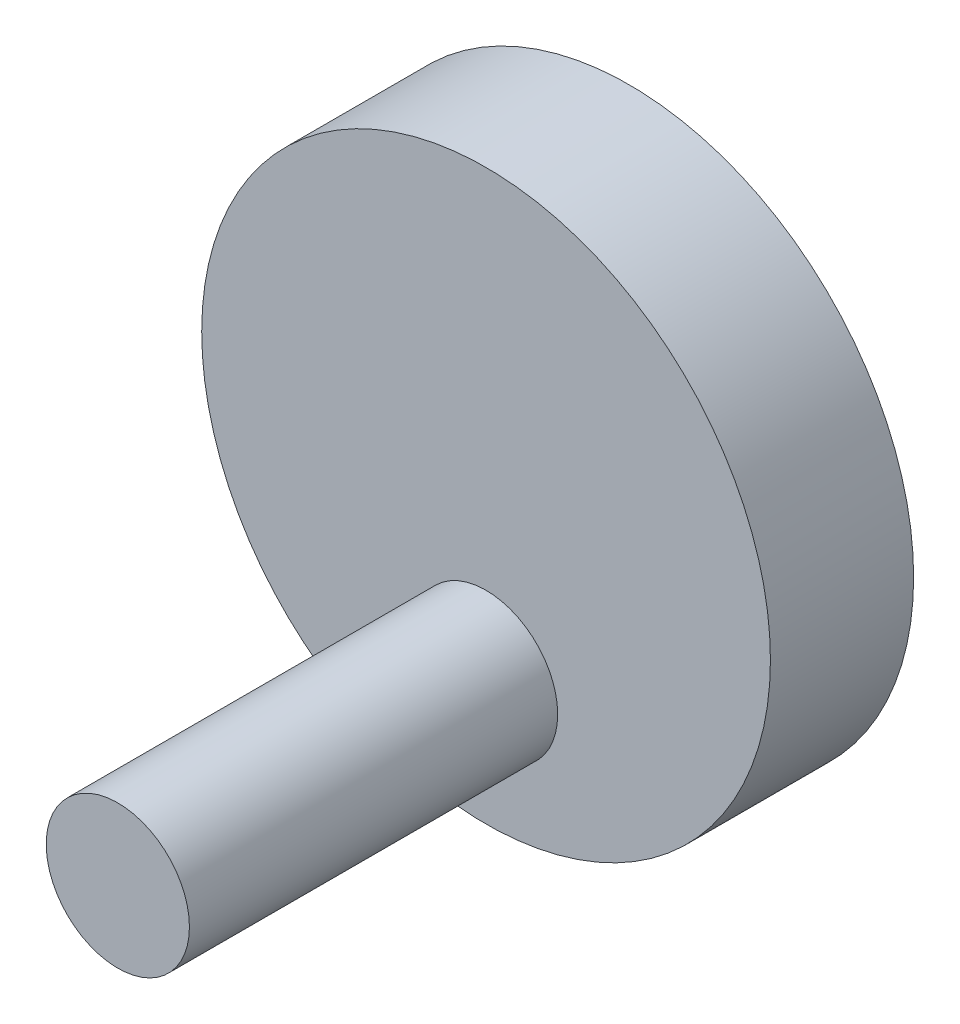
SolidWorks part; units mm, degrees
ref_plane "Front Plane" through (0, 0, 0) normal (0, 0, 1) x (1, 0, 0)
ref_plane "Top Plane" through (0, 0, 0) normal (0, 1, 0) x (1, 0, 0)
ref_plane "Right Plane" through (0, 0, 0) normal (1, 0, 0) x (0, 0, -1)
sketch "Sketch1" plane through (0, 0, 0) normal (0, 0, 1) x (1, 0, 0)
  circle A3 centre (0.6135, -35) radius 13.9
  circle A4 centre (0.6135, -35) radius 13.9
  dimension "D1" = 10
extrude "Boss-Extrude1" add sketch "Sketch1" against normal blind 5 and the other way blind 2
sketch "Sketch2" plane through (0, 0, -5) normal (0, 0, -1) x (-1, 0, 0)
  circle A0 centre (-0.6135, -35) radius 3.9 construction
  circle A1 centre (-0.6135, -35) radius 3.9
extrude "Cut-Extrude1" cut sketch "Sketch2" against normal blind 6
sketch "Sketch3" plane through (0, 0, 2) normal (0, 0, 1) x (1, 0, 0)
  line L0 (0.6135, -35) -> (0.6135, -42.5) construction
  circle A0 centre (0.6135, -42.5) radius 3.5
  dimension "D1" = 7
  dimension "D2" = 7.5
extrude "Boss-Extrude2" add sketch "Sketch3" along normal blind 18
sketch "Sketch5" plane through (0, 0, 2) normal (0, 0, 1) x (1, 0, 0)
  line L0 (0.6135, -35) -> (-5.0435, -22.3032)
  line L1 (-19.1476, -76.6473) -> (-43.5661, -21.8409) construction
  circle A0 centre (0.6135, -35) radius 13.9 construction
